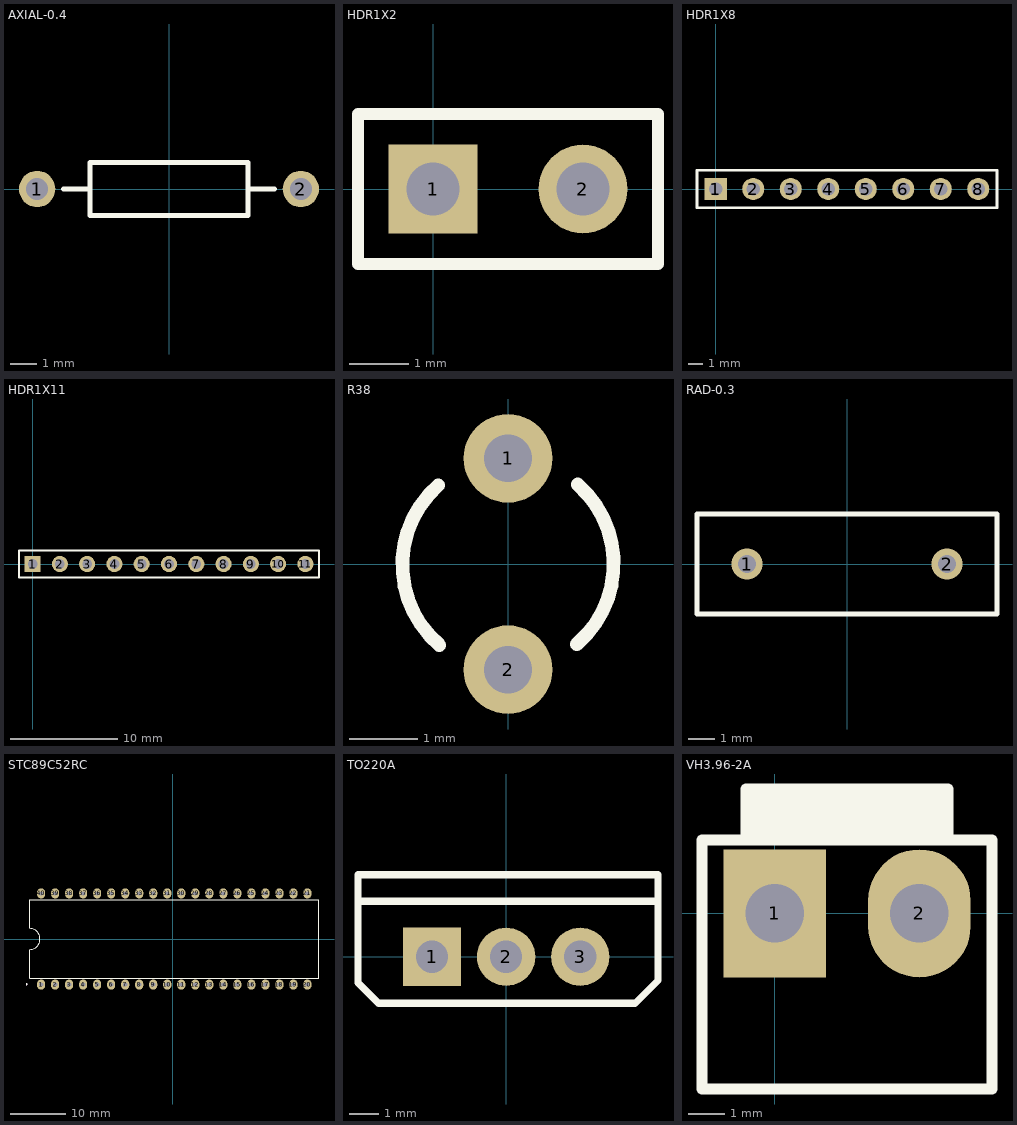
[diagram p0: the footprints below, top view; thin cyan lines are the x and y axes]
# Altium footprint library MISC82800.PcbLib: 9 footprints
Each footprint in its own frame and in the unit in brackets; x right, y up, seen from the top. Pads: shape width x height; smd on the part's side, far side on the other; paste and mask are expansions set on the pad; w line width, h text height; cw(c..) or ccw(c..) is an arc to the next point about the centre after c.

## AXIAL-0.4 [mm] "Axial Device, Thru-Hole; 2 Leads; 0.4 in Pin Spacing"
height 2.032
pads (2):
  round 1.4 hole 0.85: 1(-5.08,0) 2(5.08,0)
Top Overlay:
  lines w0.2: -4.064,0 -3.048,0 ; 3.048,0 4.064,0 ; -3.048,-1.016 -3.048,1.016 3.048,1.016 3.048,-1.016 -3.048,-1.016

## HDR1X2 [mm] "Connector; Header; 2 Position"
height 4.58
pads (2):
  rect 1.5x1.5 hole 0.9: 1(0,0)
  round 1.5 hole 0.9: 2(2.54,0)
Top Overlay:
  lines w0.2: -1.27,-1.27 -1.27,1.27 3.81,1.27 3.81,-1.27 -1.27,-1.27

## HDR1X8 [mm] "Connector; Header; 8 Position"
height 4.58
pads (8):
  rect 1.5x1.5 hole 0.9: 1(0,0)
  round 1.5 hole 0.9: 2(2.54,0) 3(5.08,0) 4(7.62,0) 5(10.16,0) 6(12.7,0) 7(15.24,0) 8(17.78,0)
Top Overlay:
  lines w0.2: -1.27,-1.27 -1.27,1.27 19.05,1.27 19.05,-1.27 -1.27,-1.27

## HDR1X11 [mm] "Connector; Header; 11 Position"
height 4.58
pads (11):
  rect 1.5x1.5 hole 0.9: 1(0,0)
  round 1.5 hole 0.9: 2(2.54,0) 3(5.08,0) 4(7.62,0) 5(10.16,0) 6(12.7,0) 7(15.24,0) 8(17.78,0) 9(20.32,0) 10(22.86,0) 11(25.4,0)
Top Overlay:
  lines w0.2: -1.27,-1.27 26.67,-1.27 26.67,1.27 0.635,1.27 -1.27,1.27 -1.27,-1.27

## R38 [mm] "Crystal, Thru-Hole; 2 Leads; Body 3.1 x 8.2 mm (Dia.xH)"
height 8.2
pads (2):
  round 1.3 hole 0.7: 1(0,1.55) 2(0,-1.55)
Top Overlay:
  lines w0.2: -1.022,1.155 ccw(c0,-0.01) -1.006,-1.189 ; 1.006,-1.179 ccw(c0,0) 1.022,1.165

## RAD-0.3 [mm] "Radial Cap, Thru-Hole; 2 Leads; 0.3 in Pin Spacing"
height 6
pads (2):
  round 1.2 hole 0.7: 1(-3.81,0) 2(3.81,0)
Top Overlay:
  lines w0.2: -5.715,-1.905 -5.715,1.905 5.715,1.905 5.715,-1.905 -5.715,-1.905

## STC89C52RC [mm]
height 4.58
pads (40):
  oval 1.467x1.833 hole 0.8 paste+0 mask+0.051: 1(-23.868,-8.255) 2(-21.328,-8.255) 3(-18.788,-8.255) 4(-16.248,-8.255) 5(-13.708,-8.255) 6(-11.168,-8.255) 7(-8.628,-8.255) 8(-6.088,-8.255) 9(-3.548,-8.255) 10(-1.008,-8.255) 11(1.532,-8.255) 12(4.072,-8.255) 13(6.612,-8.255) 14(9.152,-8.255) 15(11.692,-8.255) 16(14.232,-8.255) 17(16.772,-8.255) 18(19.312,-8.255) 19(21.852,-8.255) 20(24.392,-8.255) 21(24.392,8.255) 22(21.852,8.255) 23(19.312,8.255) 24(16.772,8.255) 25(14.232,8.255) 26(11.692,8.255) 27(9.152,8.255) 28(6.612,8.255) 29(4.072,8.255) 30(1.532,8.255) 31(-1.008,8.255) 32(-3.548,8.255) 33(-6.088,8.255) 34(-8.628,8.255) 35(-11.168,8.255) 36(-13.708,8.255) 37(-16.248,8.255) 38(-18.788,8.255) 39(-21.328,8.255) 40(-23.868,8.255)
Top Overlay:
  circle w0.15: c-26.502,-8.222 r0.075
  lines w0.152: -25.976,-7.11 26.501,-7.11 26.501,7.11 -25.976,7.11 -25.976,1.905 cw(c-25.976,0) -25.976,-1.905 -25.976,-7.11
Mechanical 15:
  circle w0.15: c-26.502,-8.222 r0.075

## TO220A [mm] "220, 3-pin transistor"
height 4.58
pads (3):
  rect 2x2 hole 1.1: 1(-2.54,0)
  round 2 hole 1.1: 2(0,0) 3(2.54,0)
Top Overlay:
  lines w0.254: -4.928,1.905 5.131,1.905 ; -5.08,-0.889 -4.369,-1.6 4.42,-1.6 5.207,-0.813 5.207,2.819 -5.08,2.819 -5.08,-0.889
3D body "4.STEP": height 18.5, standoff -4, extent -5.08,-1.453 5.22,2.977

## VH3.96-2A [mm]
height 4.58
pads (2):
  rect 2.8x3.5 hole 1.6: 1(0,0)
  oval 2.8x3.5 hole 1.6: 2(3.96,0)
Top Overlay:
  lines w0.3: -0.78,2 -0.78,3.4 4.74,3.4 4.74,2 ; -0.78,2.286 4.74,2.286 ; -0.78,2.413 4.74,2.413 ; -0.78,2.667 4.74,2.667 ; -0.78,2.921 4.74,2.921 ; -0.78,3.175 4.74,3.175 ; -1.98,-4.8 5.94,-4.8 5.94,2 -1.98,2 -1.98,-4.8
3D body "VH3.96-2A.STEP": height 14.6, standoff -3.6, extent -1.98,-4.8 5.94,3.6